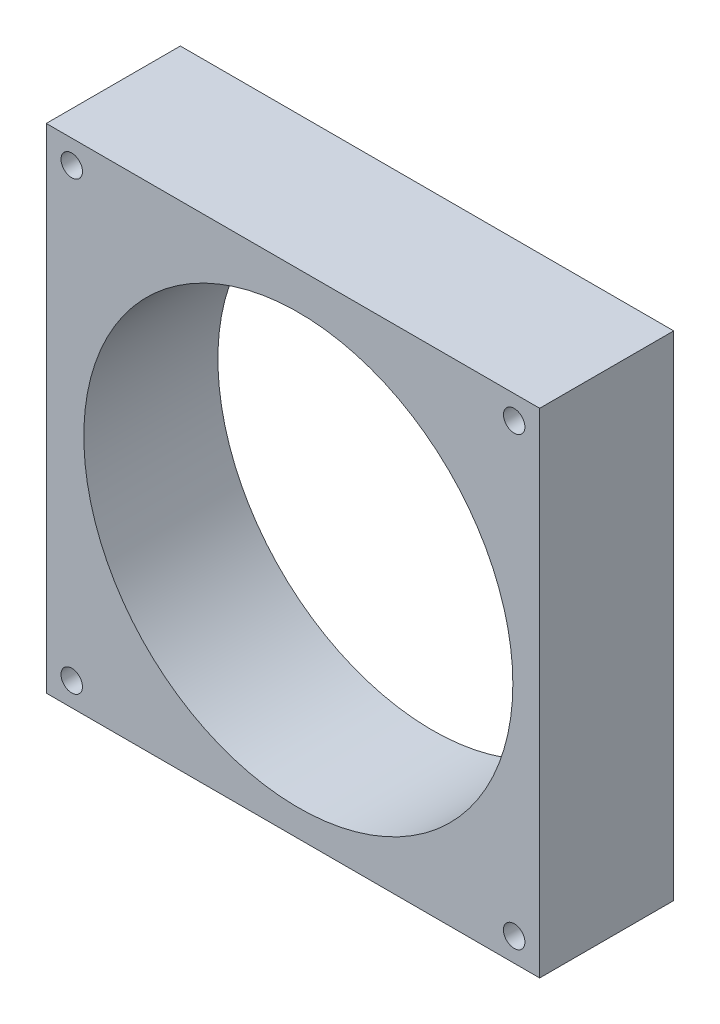
from build123d import *

# Parameters (mm, degrees)
SKETCH1_W           = 92
SKETCH1_H           = 92
BOSS_EXTRUDE1_DEPTH = 25
SKETCH2_R           = 40
CUT_EXTRUDE1_DEPTH  = 25
SKETCH3_R           = 2
CUT_EXTRUDE2_DEPTH  = 30


with BuildPart() as part:
    # Sketch1 → Boss-Extrude1 (new body)
    with BuildSketch(Plane.XY):
        with Locations((-46, 46)):
            Rectangle(SKETCH1_W, SKETCH1_H)
    extrude(amount=BOSS_EXTRUDE1_DEPTH)

    # Sketch2 → Cut-Extrude1 (cut)
    with BuildSketch(Plane.XY.offset(25)):
        with Locations((-45, 45)):
            Circle(SKETCH2_R)
    extrude(amount=-CUT_EXTRUDE1_DEPTH, mode=Mode.SUBTRACT)

    # Sketch3 → Cut-Extrude2 (cut)
    with BuildSketch(Plane.XY.offset(25)):
        with Locations((-4.75, 87.599810623)):
            Circle(SKETCH3_R)
        with Locations((-87.25, 87.599810623)):
            Circle(SKETCH3_R)
        with Locations((-87.25, 4.400189377)):
            Circle(SKETCH3_R)
        with Locations((-4.75, 4.400189377)):
            Circle(SKETCH3_R)
    extrude(amount=-CUT_EXTRUDE2_DEPTH, mode=Mode.SUBTRACT)


solid = part.part
